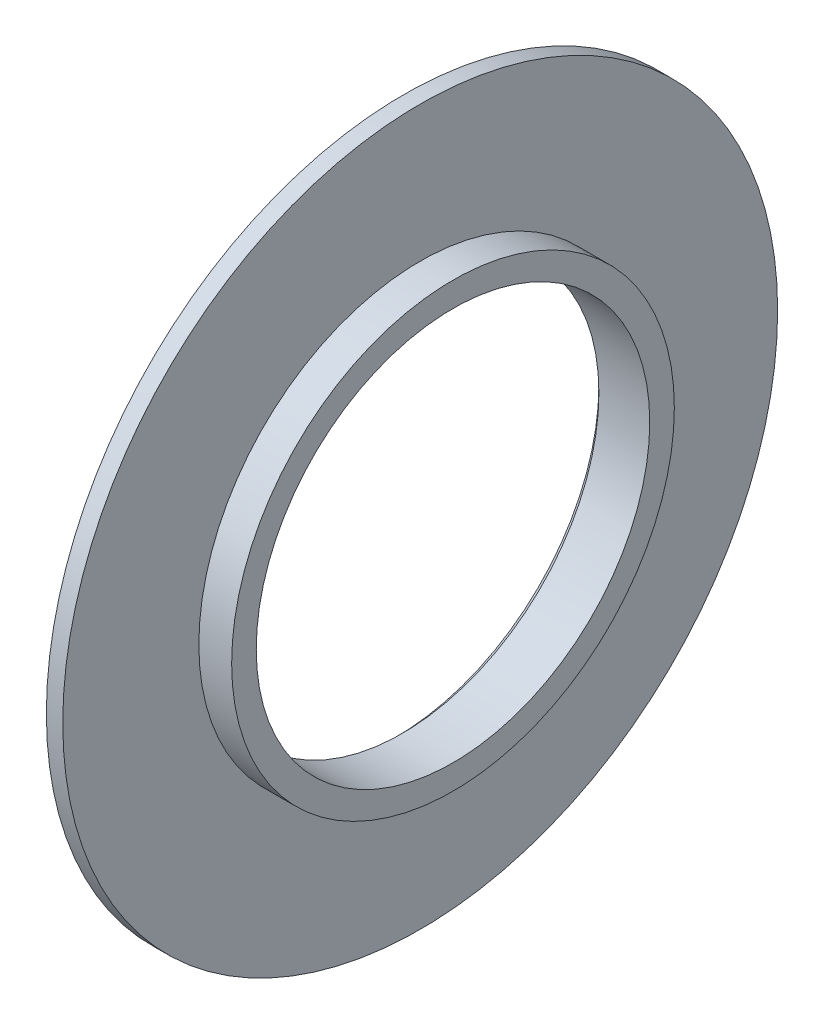
SolidWorks part; units mm, degrees
material "Q235-A"
ref_plane "Front Plane" through (0, 0, 0) normal (0, 0, 1) x (1, 0, 0)
ref_plane "Top Plane" through (0, 0, 0) normal (0, 1, 0) x (1, 0, 0)
ref_plane "Right Plane" through (0, 0, 0) normal (1, 0, 0) x (0, 0, -1)
sketch "Sketch1" plane through (0, 0, 0) normal (0, 0, 1) x (1, 0, 0)
  line L0 (0, 0) -> (256.7869, 0) construction
  line L1 (0, 140) -> (5, 140)
  line L2 (5, 140) -> (5, 218)
  line L3 (5, 218) -> (15, 218)
  line L4 (15, 218) -> (15, 135)
  line L5 (15, 135) -> (35, 135)
  line L6 (35, 135) -> (35, 120)
  line L7 (35, 120) -> (0, 120)
  line L9 (0, 120) -> (0, 140)
  dimension "D1" = 120
  dimension "D2" = 135
  dimension "D3" = 218
  dimension "D4" = 140
  dimension "D5" = 35
  dimension "D6" = 10
  dimension "D7" = 30
revolve "Revolve1" add sketch "Sketch1" angle 360 about L0
chamfer "Chamfer1" distance 4 angle 45 1 edges at (0, 0, 120)
